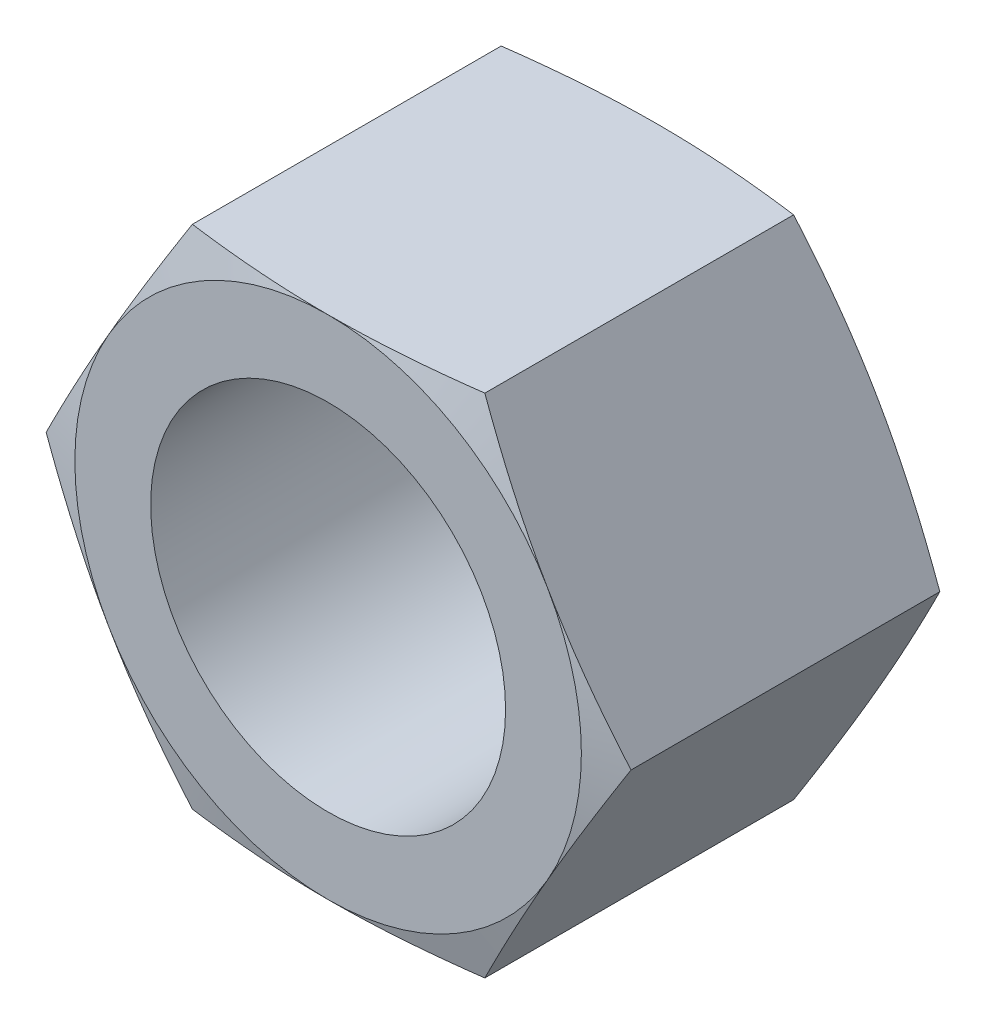
from build123d import *

# Parameters (mm, degrees)
SKETCH1_R          = 12
BASE_EXTRUDE_DEPTH = 22.3
SKETCH2_OUTSIDE_W  = 336.56
SKETCH2_OUTSIDE_H  = 331.262
SKETCH2_OUTSIDE_R  = 17.12565236
CUT_EXTRUDE1_DEPTH = 38
CUT_EXTRUDE1_DRAFT = -75
SKETCH3_OUTSIDE_W  = 336.56
SKETCH3_OUTSIDE_H  = 331.262
SKETCH3_OUTSIDE_R  = 17.12565236
CUT_EXTRUDE2_DEPTH = 38
CUT_EXTRUDE2_DRAFT = -75


with BuildPart() as part:
    # Sketch1 → Base-Extrude (new body)
    with BuildSketch(Plane.XY):
        Polygon((9.8875, 17.12565236), (-9.8875, 17.12565236), (-19.775, 0), (-9.8875, -17.12565236), (9.8875, -17.12565236), (19.775, 0), align=None)
        Circle(SKETCH1_R, mode=Mode.SUBTRACT)
    extrude(amount=BASE_EXTRUDE_DEPTH)


with BuildPart() as cut_extrude1_tool:
    # Sketch2 outside → Cut-Extrude1 (with draft: the straight prism first)
    with BuildSketch(Plane(origin=(0, 0, 0), x_dir=(-1, 0, 0), z_dir=(0, 0, -1))):
        Rectangle(SKETCH2_OUTSIDE_W, SKETCH2_OUTSIDE_H)
        Circle(SKETCH2_OUTSIDE_R, mode=Mode.SUBTRACT)
    extrude(amount=-CUT_EXTRUDE1_DEPTH)
    # Cut-Extrude1: the draft: its side faces are tilted about the plane it starts from
    cut_extrude1_sides = [cut_extrude1_tool.faces().sort_by_distance(p)[0] for p in [
        (0, -165.631, 19),
        (-168.28, 0, 19),
        (0, 165.631, 19),
        (168.28, 0, 19),
        (17.12565236, 0, 19),
    ]]
    draft(cut_extrude1_sides, Plane(origin=(0, 0, 0), x_dir=(-1, 0, 0), z_dir=(0, 0, -1)), CUT_EXTRUDE1_DRAFT)


with BuildPart() as part_1:
    add(part.part)

    # Cut-Extrude1: cut by cut_extrude1_tool
    add(cut_extrude1_tool.part, mode=Mode.SUBTRACT)


with BuildPart() as cut_extrude2_tool:
    # Sketch3 outside → Cut-Extrude2 (with draft: the straight prism first)
    with BuildSketch(Plane.XY.offset(22.3)):
        Rectangle(SKETCH3_OUTSIDE_W, SKETCH3_OUTSIDE_H)
        Circle(SKETCH3_OUTSIDE_R, mode=Mode.SUBTRACT)
    extrude(amount=-CUT_EXTRUDE2_DEPTH)
    # Cut-Extrude2: the draft: its side faces are tilted about the plane it starts from
    cut_extrude2_sides = [cut_extrude2_tool.faces().sort_by_distance(p)[0] for p in [
        (0, -165.631, 3.3),
        (168.28, 0, 3.3),
        (0, 165.631, 3.3),
        (-168.28, 0, 3.3),
        (-17.12565236, 0, 3.3),
    ]]
    draft(cut_extrude2_sides, Plane.XY.offset(22.3), CUT_EXTRUDE2_DRAFT)


with BuildPart() as part_2:
    add(part_1.part)

    # Cut-Extrude2: cut by cut_extrude2_tool
    add(cut_extrude2_tool.part, mode=Mode.SUBTRACT)


solid = part_2.part
